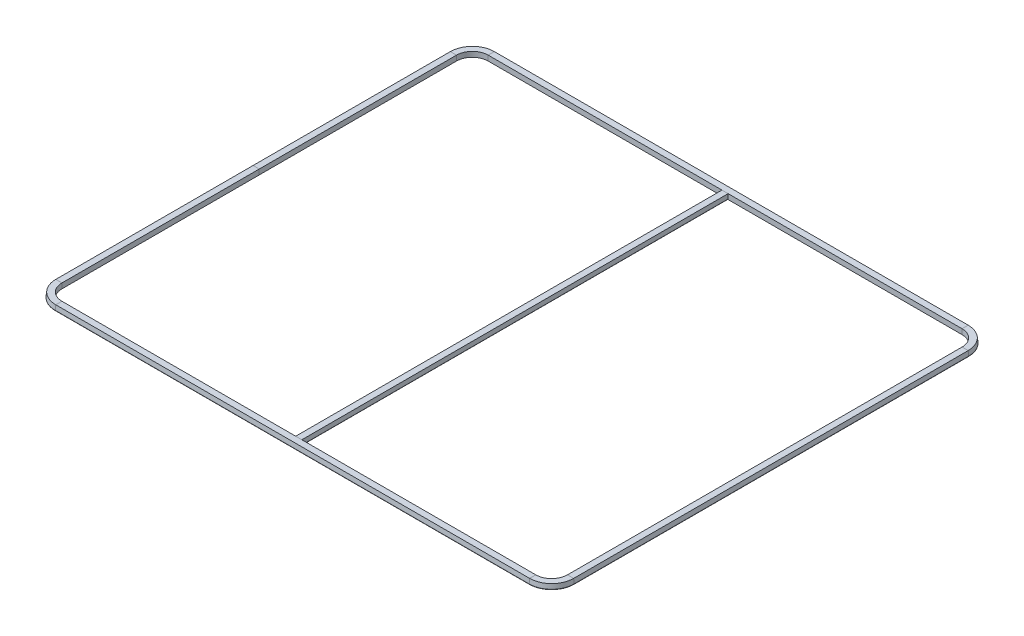
from build123d import *

# Parameters (mm, degrees)
EXTRUDE_1_REACH             = 1717.304
EXTRUDE_1_DIRECTION_2_REACH = 1717.304
FILLET_1_R                  = 3


with BuildPart() as part:
    # 扫描1: sweep along a path in 草图1
    with BuildLine(Plane(origin=(0, 0, 0), x_dir=(1, 0, 0), z_dir=(0, 1, 0))) as sweep_1_path:
        Line((-1195, -1090), (1195, -1090))
        ThreePointArc((1195, -1090), (1262.175144213, -1062.175144213), (1290, -995))
        Line((1290, -995), (1290, 995))
        ThreePointArc((1290, 995), (1262.175144213, 1062.175144213), (1195, 1090))
        Line((1195, 1090), (-1195, 1090))
        ThreePointArc((-1195, 1090), (-1262.175144213, 1062.175144213), (-1290, 995))
        Line((-1290, 995), (-1290, -995))
        ThreePointArc((-1290, -995), (-1262.175144213, -1062.175144213), (-1195, -1090))
    # 草图2 → 扫描1 (sweep)
    with BuildSketch(Plane.XY):
        with BuildLine():
            Line((-1275, 0), (-1305.63394177, 0))
            ThreePointArc((-1305.63394177, 0), (-1307.873541843, 1.003956034), (-1308.614168578, 3.343872324))
            Line((-1308.614168578, 3.343872324), (-1306, 26))
            Line((-1306, 26), (-1275, 26))
            Line((-1275, 26), (-1275, 0))
        make_face()
    sweep(path=sweep_1_path.line)


with BuildPart() as body_2:

    # 草图3 → 凸台-拉伸1 (new, up to next)
    with BuildSketch(Plane.XY, mode=Mode.PRIVATE) as extrude_1_sk1:
        Polygon((-16, 26), (-19, 0), (15, 0), (15, 26), align=None)
    extrude_1_tool1 = extrude(extrude_1_sk1.sketch, amount=EXTRUDE_1_REACH, mode=Mode.PRIVATE) - part.part
    add(extrude_1_tool1.solids().sort_by_distance((-1.261538, 12.8, 0))[0])


    # 草图3 → 凸台-拉伸1 direction 2 (add, up to next)
    with BuildSketch(Plane.XY, mode=Mode.PRIVATE) as extrude_1_direction_2_sk1:
        Polygon((-16, 26), (-19, 0), (15, 0), (15, 26), align=None)
    extrude_1_direction_2_tool1 = extrude(extrude_1_direction_2_sk1.sketch, amount=-EXTRUDE_1_DIRECTION_2_REACH, mode=Mode.PRIVATE) - part.part
    add(extrude_1_direction_2_tool1.solids().sort_by_distance((-1.261538, 12.8, 0))[0])

    # 圆角1
    fillet_1_edges = [body_2.edges().sort_by_distance(p)[0] for p in [
        (15, 0, 0),
        (-19, 0, 0),
    ]]
    fillet(fillet_1_edges, radius=FILLET_1_R)


solid = Compound([part.part, body_2.part])
